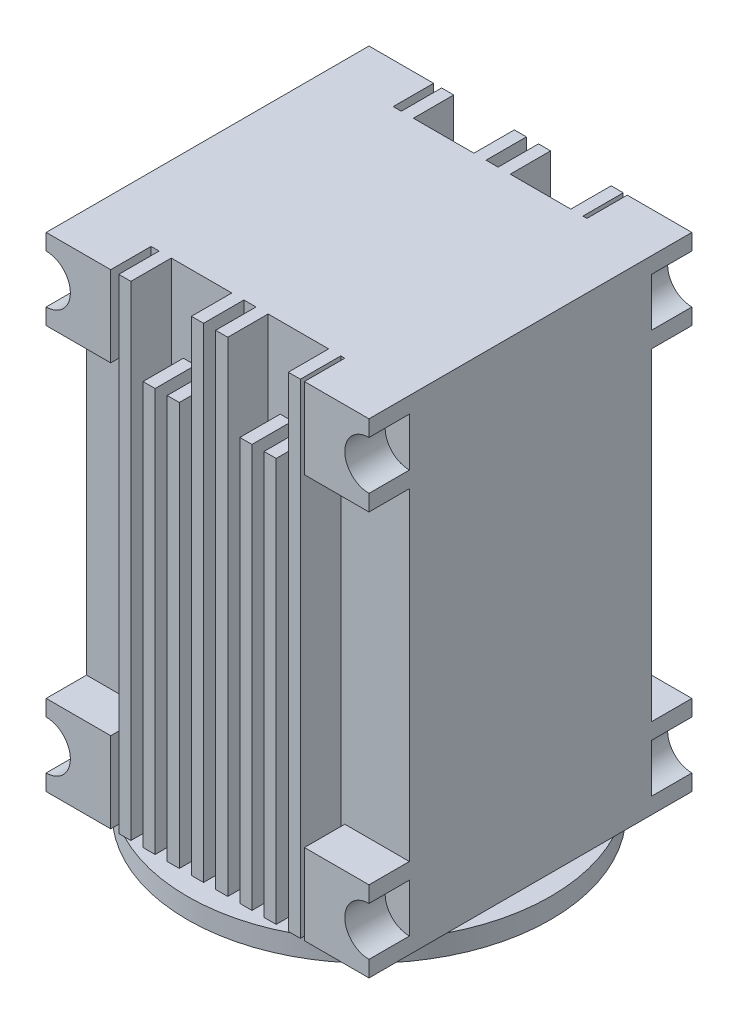
SolidWorks part; units mm, degrees
ref_plane "Front Plane" through (0, 0, 0) normal (0, 0, 1) x (1, 0, 0)
ref_plane "Top Plane" through (0, 0, 0) normal (0, 1, 0) x (1, 0, 0)
ref_plane "Right Plane" through (0, 0, 0) normal (1, 0, 0) x (0, 0, -1)
other "Configuration Table"
sketch "Sketch1" plane through (0, 0, 0) normal (0, 1, 0) x (1, 0, 0)
  line L1 (-20, -20) -> (20, -20)
  line L2 (-20, -20) -> (-20, 20)
  line L3 (-20, 20) -> (20, 20)
  line L4 (20, -20) -> (20, 20)
  line L5 (-20, -20) -> (20, 20) construction
  line L6 (-20, 20) -> (20, -20) construction
  point P0 (0, 0)
  dimension "D1" = 40
  dimension "D2" = 40
extrude "Boss-Extrude1" add sketch "Sketch1" along normal mid plane 60
sketch "Sketch2" plane through (0, 0, -20) normal (0, 0, -1) x (-1, 0, 0)
  line L0 (-12, 30) -> (12, 30)
  line L1 (-20, 30) -> (-12, 30) construction
  line L2 (-20, 30) -> (-20, 20) construction
  line L3 (-20, 20) -> (-12, 20)
  line L4 (-12, 30) -> (-12, 20)
  line L5 (20, 30) -> (12, 30) construction
  line L6 (20, 30) -> (20, 20) construction
  line L7 (20, 20) -> (12, 20)
  line L8 (12, 30) -> (12, 20)
  line L9 (-20, -30) -> (-12, -30) construction
  line L10 (-20, -30) -> (-20, -20) construction
  line L11 (-20, -20) -> (-12, -20)
  line L12 (-12, -30) -> (-12, -20)
  line L13 (20, -30) -> (12, -30) construction
  line L14 (20, -30) -> (20, -20) construction
  line L15 (20, -20) -> (12, -20)
  line L16 (12, -30) -> (12, -20)
  line L17 (-20, 20) -> (-20, -20)
  line L18 (-12, -30) -> (12, -30)
  line L19 (20, 20) -> (20, -20)
  dimension "D1" = 8
  dimension "D2" = 10
  dimension "D3" = 10
  dimension "D4" = 10
  dimension "D5" = 10
  dimension "D6" = 8
extrude "Cut-Extrude1" cut sketch "Sketch2" against normal blind 5
mirror "Mirror1" about plane through (0, 0, 0) normal (0, 0, 1) of "Cut-Extrude1"
sketch "Sketch3" plane through (0, 30, 0) normal (0, 1, 0) x (1, 0, 0)
  line L0 (-12, 15) -> (12, 15) construction
  line L1 (-11, 15) -> (-9.5, 15)
  line L2 (-11, 15) -> (-11, 20)
  line L3 (-11, 20) -> (-9.5, 20)
  line L4 (-9.5, 15) -> (-9.5, 20)
  line L5 (-12, 15) -> (-12, 20) construction
  line L6 (0, 0) -> (10.5943, 0) construction
  line L7 (-8, 20) -> (-6.5, 20)
  line L8 (-8, 15) -> (-8, 20)
  line L9 (-6.5, 15) -> (-6.5, 20)
  line L10 (-8, 15) -> (-6.5, 15)
  line L11 (-5, 20) -> (-3.5, 20)
  line L12 (-5, 15) -> (-5, 20)
  line L13 (-3.5, 15) -> (-3.5, 20)
  line L14 (-5, 15) -> (-3.5, 15)
  line L15 (-2, 20) -> (-0.5, 20)
  line L16 (-2, 15) -> (-2, 20)
  line L17 (-0.5, 15) -> (-0.5, 20)
  line L18 (-2, 15) -> (-0.5, 15)
  line L19 (1, 20) -> (2.5, 20)
  line L20 (1, 15) -> (1, 20)
  line L21 (2.5, 15) -> (2.5, 20)
  line L22 (1, 15) -> (2.5, 15)
  line L23 (4, 20) -> (5.5, 20)
  line L24 (4, 15) -> (4, 20)
  line L25 (5.5, 15) -> (5.5, 20)
  line L26 (4, 15) -> (5.5, 15)
  line L27 (7, 20) -> (8.5, 20)
  line L28 (7, 15) -> (7, 20)
  line L29 (8.5, 15) -> (8.5, 20)
  line L30 (7, 15) -> (8.5, 15)
  line L31 (10, 20) -> (11.5, 20)
  line L32 (10, 15) -> (10, 20)
  line L33 (11.5, 15) -> (11.5, 20)
  line L34 (10, 15) -> (11.5, 15)
  dimension "D1" = 1
  dimension "D2" = 1.5
  dimension "D4" = 3
  dimension "D3" = 8
extrude "Boss-Extrude2" add sketch "Sketch3" against normal up to surface (60 mm away) up to face at (0, -30, 0)
sketch "Sketch4" plane through (0, 0, -20) normal (0, 0, -1) x (-1, 0, 0)
  line L0 (-4, -30) -> (-4, 30) construction
  line L1 (-8.5, 30) -> (-4, 30)
  line L2 (-8.5, 30) -> (-8.5, 20)
  line L3 (-8.5, 20) -> (-4, 20)
  line L4 (-4, 30) -> (-4, 20)
  line L5 (8, -30) -> (8, 30) construction
  line L6 (3.5, 30) -> (8, 30)
  line L7 (3.5, 30) -> (3.5, 20)
  line L8 (3.5, 20) -> (8, 20)
  line L9 (8, 30) -> (8, 20)
  dimension "D1" = 10
extrude "Cut-Extrude2" cut sketch "Sketch4" against normal blind 5
mirror "Mirror2" about plane through (0, 0, 0) normal (0, 0, 1) of "Cut-Extrude2", "Boss-Extrude2"
sketch "Sketch5" plane through (0, 0, -20) normal (0, 0, -1) x (-1, 0, 0)
  line L0 (-20, 30) -> (-20, 20) construction
  line L2 (0, 0) -> (0, 10.117) construction
  line L3 (0, 0) -> (16.5103, 0) construction
  circle A1 centre (-20, 25) radius 3
  circle A2 centre (20, 25) radius 3
  circle A3 centre (-20, -25) radius 3
  circle A4 centre (20, -25) radius 3
  dimension "D1" = 6
extrude "Cut-Extrude3" cut sketch "Sketch5" against normal blind 5
mirror "Mirror3" about plane through (0, 0, 0) normal (0, 0, 1) of "Cut-Extrude3"
sketch "Sketch6" plane through (0, -30, 0) normal (0, -1, 0) x (1, 0, 0)
  circle A0 centre (0, 0) radius 22.5
  dimension "D1" = 45
extrude "Boss-Extrude3" add sketch "Sketch6" along normal blind 2.5 contours A0
sketch "Sketch7" plane through (0, -32.5, 0) normal (0, -1, 0) x (1, 0, 0)
  circle A0 centre (0, 0) radius 5
  dimension "D1" = 10
extrude "Cut-Extrude4" cut sketch "Sketch7" against normal blind 15 contours A0
sketch "Sketch8" plane through (-20, 0, 0) normal (-1, 0, 0) x (0, 0, 1)
  line L0 (-20, 30) -> (20, 30) construction
  circle A0 centre (4.37, 17.51) radius 2.5
  dimension "D3" = 5
  dimension "D1" = 24.37
  dimension "D2" = 12.49
extrude "Cut-Extrude6" cut sketch "Sketch8" against normal blind 15 contours A0
sketch "Sketch9" plane through (0, -30, 0) normal (0, -1, 0) x (1, 0, 0)
  line L0 (-20, -20) -> (-20, -10.3078) construction
  line L1 (-12, -20) -> (-20, -20) construction
  line L2 (20, -10.3078) -> (20, -20) construction
  line L3 (12, 20) -> (20, 20) construction
  circle A0 centre (-17.5, 17.5) radius 1
  circle A1 centre (-17.5, -17.5) radius 1
  circle A2 centre (17.5, -17.5) radius 1
  circle A3 centre (17.5, 17.5) radius 1
  dimension "D1" = 2
  dimension "D2" = 2
  dimension "D3" = 2
  dimension "D4" = 2
  dimension "D5" = 2.5
  dimension "D6" = 2.5
  dimension "D7" = 2.5
  dimension "D8" = 2.5
extrude "Cut-Extrude7" cut sketch "Sketch9" against normal blind 1.8
